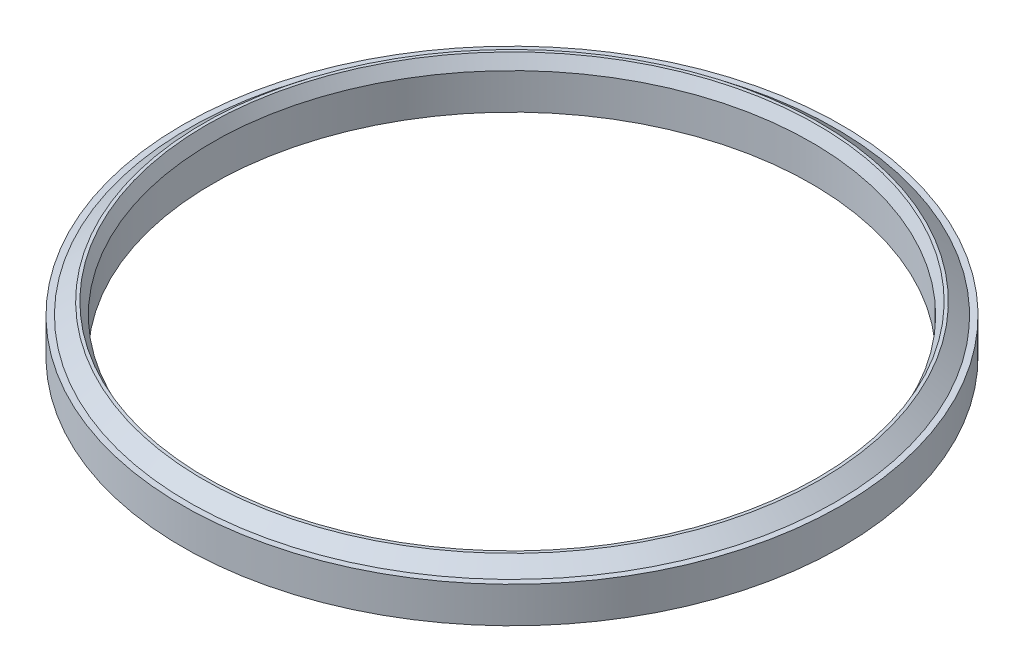
SolidWorks part; units mm, degrees
material "6061-T6 (SS)"
ref_plane "Front Plane" through (0, 0, 0) normal (0, 0, 1) x (1, 0, 0)
ref_plane "Top Plane" through (0, 0, 0) normal (0, 1, 0) x (1, 0, 0)
ref_plane "Right Plane" through (0, 0, 0) normal (1, 0, 0) x (0, 0, -1)
sketch "Sketch2" plane through (0, 0, 0) normal (0, 0, 1) x (1, 0, 0)
  line L0 (0, -1000) -> (0, 49000) construction
  line L1 (50, 0) -> (55, 0)
  line L2 (55, 0) -> (55, 6)
  line L3 (55, 6) -> (54, 6)
  line L4 (54, 6) -> (51.5, 8)
  line L5 (51.5, 8) -> (51, 8)
  line L6 (51, 8) -> (50, 6)
  line L7 (50, 6) -> (50, 0)
  dimension "D1" = 100
  dimension "D2" = 110
  dimension "D3" = 6
  dimension "D4" = 0.5
  dimension "D5" = 8
  dimension "D6" = 102
  dimension "D7" = 108
revolve "Revolve1" add sketch "Sketch2" angle 360 about L0
